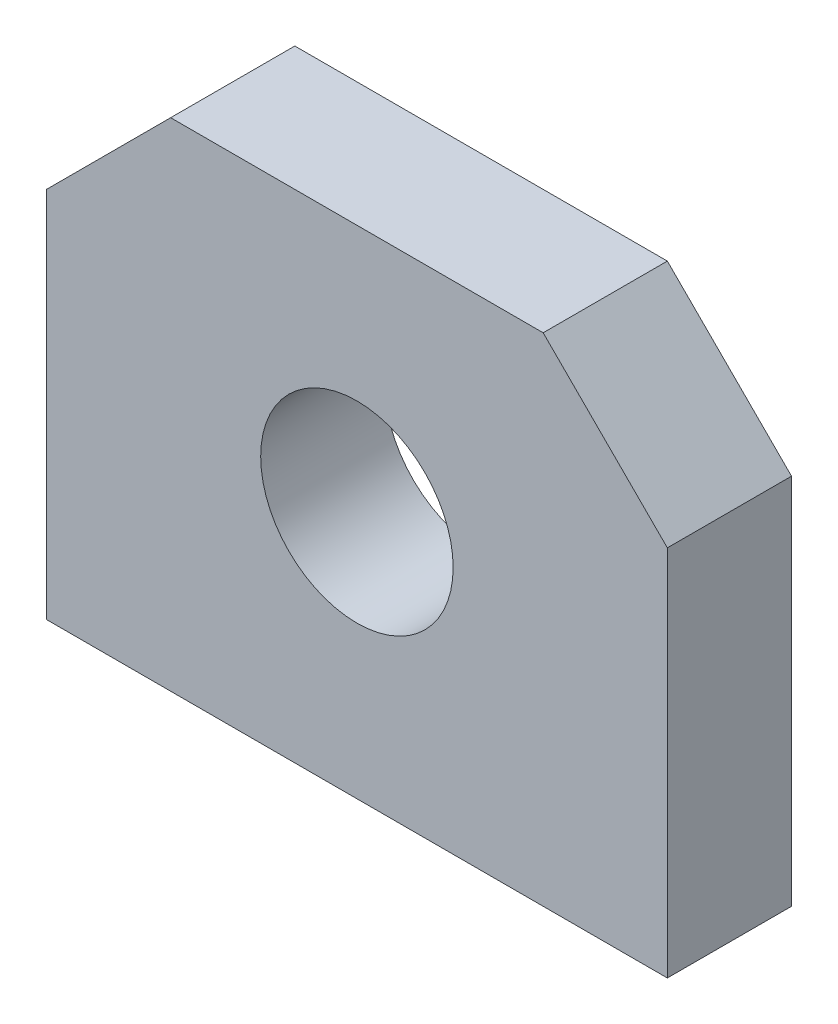
from build123d import *

# Parameters (mm, degrees)
SKETCH1_W              = 50
SKETCH1_H              = 40
BOSS_EXTRUDE1_DEPTH    = 10
CHAMFER1_SIZE          = 10
M18_TAPPED_HOLE1_D     = 15.5
M18_TAPPED_HOLE1_DEPTH = 43.5
M18_TAPPED_HOLE1_TIP   = 4.656669797


with BuildPart() as part:
    # Sketch1 → Boss-Extrude1 (new body)
    with BuildSketch(Plane.XY):
        Rectangle(SKETCH1_W, SKETCH1_H)
    extrude(amount=BOSS_EXTRUDE1_DEPTH)

    # Chamfer1
    chamfer1_edges = [part.edges().sort_by_distance(p)[0] for p in [
        (25, 20, 5),
        (-25, 20, 5),
    ]]
    chamfer(chamfer1_edges, length=CHAMFER1_SIZE)

    # M18 Tapped Hole1
    with Locations(Plane(origin=(0, 0, 0), x_dir=(-1, 0, 0), z_dir=(0, 0, -1))):
        with Locations((0, 0)):
            Hole(M18_TAPPED_HOLE1_D / 2, depth=M18_TAPPED_HOLE1_DEPTH)
            with Locations((0, 0, -(M18_TAPPED_HOLE1_DEPTH + M18_TAPPED_HOLE1_TIP / 2))):  # 118° drill point
                Cone(0, M18_TAPPED_HOLE1_D / 2, M18_TAPPED_HOLE1_TIP, mode=Mode.SUBTRACT)


solid = part.part
